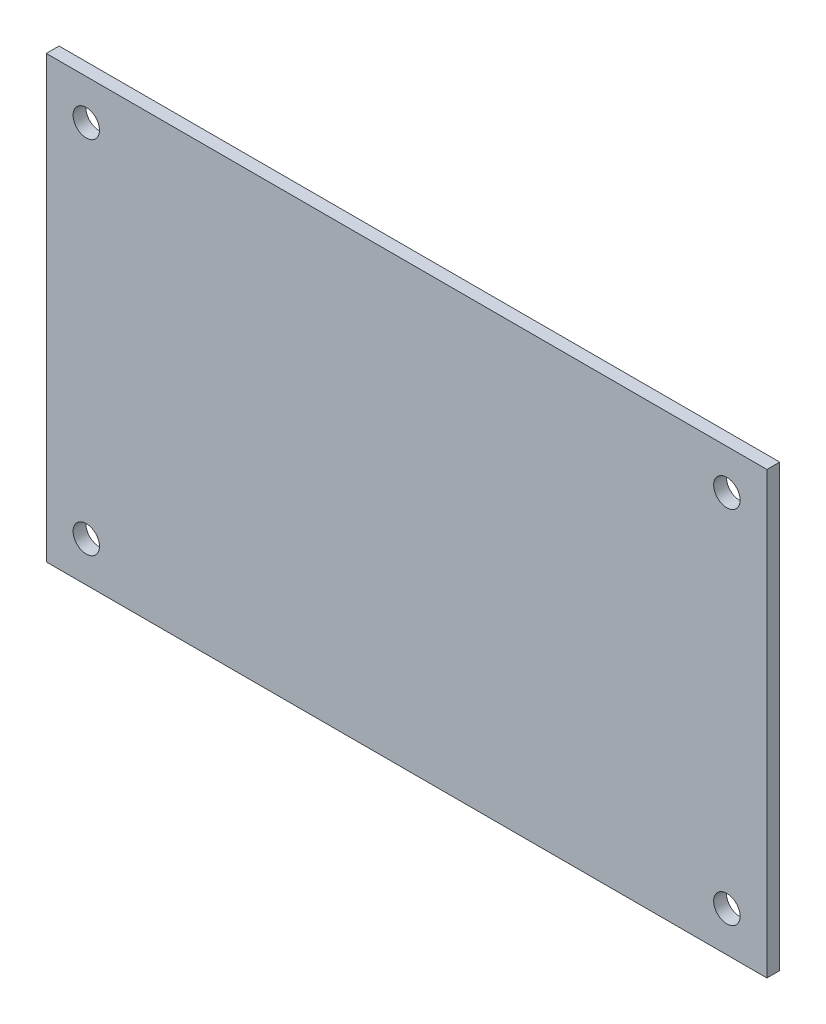
from build123d import *

# Parameters (mm, degrees)
SKETCH_1_W      = 90
SKETCH_1_H      = 55
SKETCH_1_R      = 1.65
EXTRUDE_1_DEPTH = 0.8


with BuildPart() as part:
    # 草图1 → 凸台-拉伸1 (new, symmetric)
    with BuildSketch(Plane.XY):
        Rectangle(SKETCH_1_W, SKETCH_1_H)
        with Locations((-40, -22.5)):
            Circle(SKETCH_1_R, mode=Mode.SUBTRACT)
        with Locations((-40, 22.5)):
            Circle(SKETCH_1_R, mode=Mode.SUBTRACT)
        with Locations((40, -22.5)):
            Circle(SKETCH_1_R, mode=Mode.SUBTRACT)
        with Locations((40, 22.5)):
            Circle(SKETCH_1_R, mode=Mode.SUBTRACT)
    extrude(amount=EXTRUDE_1_DEPTH, both=True)


solid = part.part
